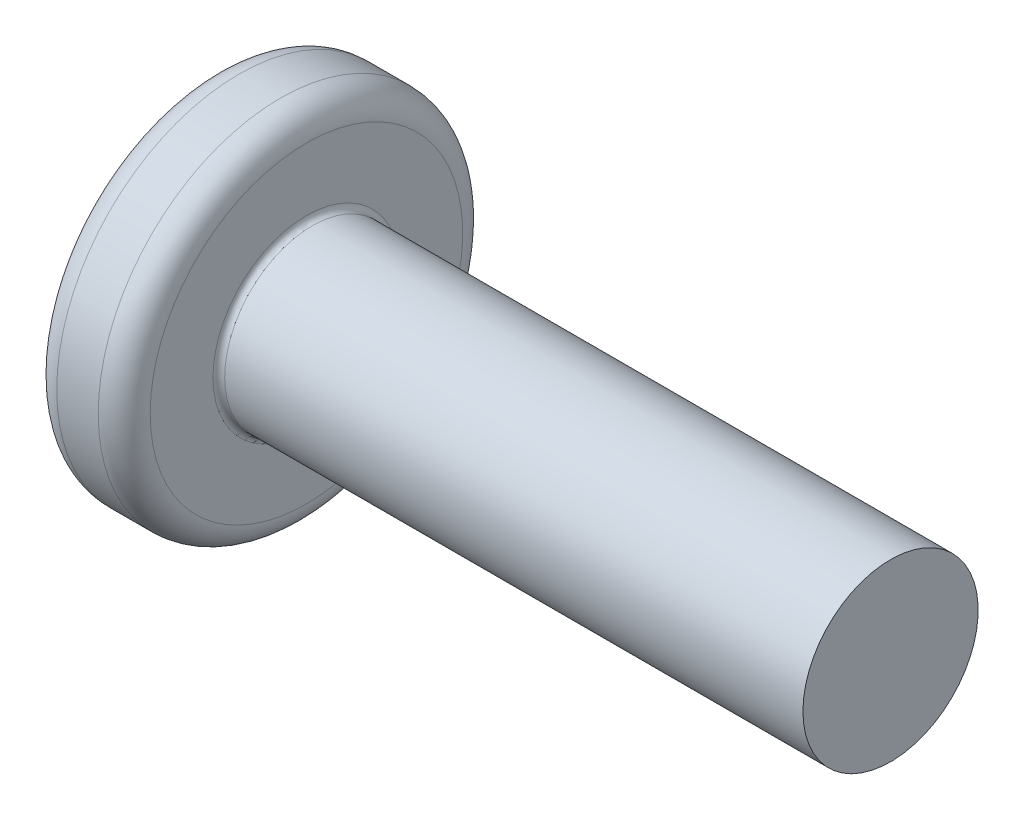
from build123d import *


with BuildPart() as part:
    # Dimensioned Sketch → Revolve3 (revolve)
    with BuildSketch(Plane.XY, mode=Mode.PRIVATE) as revolve3_sk:
        with BuildLine():
            Line((0, 0), (0, 2.6752))
            ThreePointArc((0, 2.6752), (0.130278904, 2.989721096), (0.4448, 3.12))
            Line((0.4448, 3.12), (1.1552, 3.12))
            ThreePointArc((1.1552, 3.12), (1.469721096, 2.989721096), (1.6, 2.6752))
            Line((1.6, 2.6752), (1.6, 1.6))
            ThreePointArc((1.6, 1.6), (1.629289322, 1.529289322), (1.7, 1.5))
            Line((1.7, 1.5), (11.6, 1.5))
            Line((11.6, 1.5), (11.6, 0))
            Line((11.6, 0), (0, 0))
        make_face()
    revolve(revolve3_sk.sketch.rotate(Axis((0, 0, 0), (1, 0, 0)), 90), axis=Axis((0, 0, 0), (1, 0, 0)))


solid = part.part
